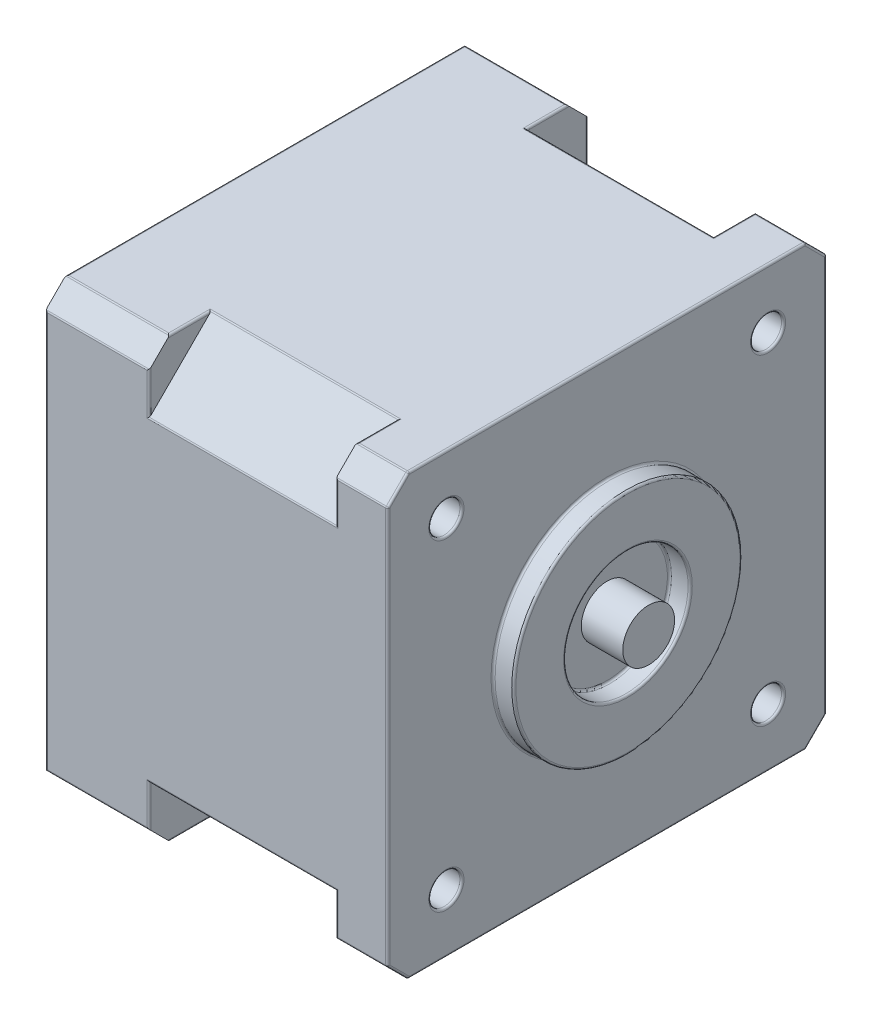
from build123d import *

# Parameters (mm, degrees)
BOSS_EXTRUDE1_DEPTH            = 5
BOSS_EXTRUDE2_DEPTH            = 18
BOSS_EXTRUDE3_DEPTH            = 10
BOSS_EXTRUDE4_DEPTH            = 2
SKETCH5_R                      = 11
BOSS_EXTRUDE5_DEPTH            = 2
F_12_0_12_DIAMETER_HOLE1_D     = 12.000000009
F_12_0_12_DIAMETER_HOLE1_DEPTH = 2
SKETCH8_W                      = 0.75
SKETCH8_H                      = 8
SKETCH9_W                      = 0.75
SKETCH9_H                      = 8
SKETCH10_W                     = 0.75
SKETCH10_H                     = 8
SKETCH11_W                     = 0.75
SKETCH11_H                     = 8
SKETCH12_W                     = 0.75
SKETCH12_H                     = 8
SKETCH13_W                     = 26
SKETCH13_H                     = 2.5
F_3_0_3_DIAMETER_HOLE1_D       = 2.999999994
F_3_0_3_DIAMETER_HOLE1_DEPTH   = 4.5
FILLET1_R                      = 0.2
SKETCH16_R                     = 3.097425191
CUT_EXTRUDE1_DEPTH             = 22


with BuildPart() as part:
    # Sketch1 → Boss-Extrude1 (new body)
    with BuildSketch(Plane(origin=(16.5, 0, 0), x_dir=(0, 0, -1), z_dir=(1, 0, 0))):
        Polygon((-21.15, 19.15), (-21.15, -19.15), (-19.15, -21.15), (19.15, -21.15), (21.15, -19.15), (21.15, 19.15), (19.15, 21.15), (-19.15, 21.15), align=None)
    extrude(amount=-BOSS_EXTRUDE1_DEPTH)

    # Sketch2 → Boss-Extrude2 (add)
    with BuildSketch(Plane.ZY.offset(-11.5)):
        Polygon((-15.15, 21.15), (15.15, 21.15), (21.15, 15.15), (21.15, -15.15), (15.15, -21.15), (-15.15, -21.15), (-21.15, -15.15), (-21.15, 15.15), align=None)
    extrude(amount=BOSS_EXTRUDE2_DEPTH)

    # Sketch3 → Boss-Extrude3 (add)
    with BuildSketch(Plane.ZY.offset(6.5)):
        Polygon((-19.15, -21.15), (-21.15, -19.15), (-21.15, 19.15), (-19.15, 21.15), (19.15, 21.15), (21.15, 19.15), (21.15, -19.15), (19.15, -21.15), align=None)
    extrude(amount=BOSS_EXTRUDE3_DEPTH)

    # Sketch4 → Boss-Extrude4 (add)
    with BuildSketch(Plane.XZ.offset(21.15)):
        with BuildLine():
            Line((-9.5, -5), (-14.5, -5))
            Line((-14.5, -5), (-14.5, 5))
            Line((-14.5, 5), (-9.5, 5))
            ThreePointArc((-9.5, 5), (-4.5, 0), (-9.5, -5))
        make_face()
    extrude(amount=BOSS_EXTRUDE4_DEPTH)

    # Sketch5 → Boss-Extrude5 (add)
    with BuildSketch(Plane(origin=(16.5, 0, 0), x_dir=(0, 0, -1), z_dir=(1, 0, 0))):
        Circle(SKETCH5_R)
    extrude(amount=BOSS_EXTRUDE5_DEPTH)

    # Ø12.0 (12) Diameter Hole1
    with Locations(Plane(origin=(18.5, 0, 0), x_dir=(0, 0, -1), z_dir=(1, 0, 0))):
        with Locations((0, 0)):
            Hole(F_12_0_12_DIAMETER_HOLE1_D / 2, depth=F_12_0_12_DIAMETER_HOLE1_DEPTH)

    # Sketch8 → Revolve1 (revolve)
    with BuildSketch(Plane.XY.offset(-4), mode=Mode.PRIVATE) as revolve1_sk:
        with Locations((-9.125, -27.15)):
            Rectangle(SKETCH8_W, SKETCH8_H)
    revolve(revolve1_sk.sketch.rotate(Axis((-9.5, -23.15, -4), (0, -1, 0)), 270), axis=Axis((-9.5, -23.15, -4), (0, -1, 0)))

    # Sketch9 → Revolve2 (revolve)
    with BuildSketch(Plane.XY.offset(-2), mode=Mode.PRIVATE) as revolve2_sk:
        with Locations((-9.125, -27.15)):
            Rectangle(SKETCH9_W, SKETCH9_H)
    revolve(revolve2_sk.sketch.rotate(Axis((-9.5, -23.15, -2), (0, -1, 0)), 270), axis=Axis((-9.5, -23.15, -2), (0, -1, 0)))

    # Sketch10 → Revolve3 (revolve)
    with BuildSketch(Plane.XY.offset(4), mode=Mode.PRIVATE) as revolve3_sk:
        with Locations((-9.125, -27.15)):
            Rectangle(SKETCH10_W, SKETCH10_H)
    revolve(revolve3_sk.sketch.rotate(Axis((-9.5, -23.15, 4), (0, -1, 0)), 270), axis=Axis((-9.5, -23.15, 4), (0, -1, 0)))

    # Sketch11 → Revolve4 (revolve)
    with BuildSketch(Plane.XY.offset(2), mode=Mode.PRIVATE) as revolve4_sk:
        with Locations((-9.125, -27.15)):
            Rectangle(SKETCH11_W, SKETCH11_H)
    revolve(revolve4_sk.sketch.rotate(Axis((-9.5, -23.15, 2), (0, -1, 0)), 270), axis=Axis((-9.5, -23.15, 2), (0, -1, 0)))

    # Sketch12 → Revolve5 (revolve)
    with BuildSketch(Plane.XY, mode=Mode.PRIVATE) as revolve5_sk:
        with Locations((-9.125, -27.15)):
            Rectangle(SKETCH12_W, SKETCH12_H)
    revolve(revolve5_sk.sketch.rotate(Axis((-9.5, -23.15, 0), (0, -1, 0)), 270), axis=Axis((-9.5, -23.15, 0), (0, -1, 0)))

    # Sketch13 → Revolve6 (revolve)
    with BuildSketch(Plane.XY, mode=Mode.PRIVATE) as revolve6_sk:
        with Locations((29.5, 1.25)):
            Rectangle(SKETCH13_W, SKETCH13_H)
    revolve(revolve6_sk.sketch.rotate(Axis((16.5, 0, 0), (1, 0, 0)), 270), axis=Axis((16.5, 0, 0), (1, 0, 0)))

    # Ø3.0 (3) Diameter Hole1
    with Locations(Plane(origin=(16.5, 0, 0), x_dir=(0, 0, -1), z_dir=(1, 0, 0))):
        with Locations((-15.5, 15.5), (15.5, -15.5), (15.5, 15.5), (-15.5, -15.5)):
            Hole(F_3_0_3_DIAMETER_HOLE1_D / 2, depth=F_3_0_3_DIAMETER_HOLE1_DEPTH)

    # Fillet1
    fillet1_edges = [part.edges().sort_by_distance(p)[0] for p in [
        (-16.5, 21.15, 0),
        (-11.5, 21.15, -19.15),
        (-11.5, 21.15, 19.15),
        (-6.5, 21.15, -17.15),
        (-11.5, 19.15, -21.15),
        (-16.5, 0, -21.15),
        (-16.5, 0, 21.15),
        (-6.5, 21.15, 17.15),
        (-11.5, 19.15, 21.15),
        (2.5, 21.15, -15.15),
        (-6.5, 17.15, -21.15),
        (-11.5, -19.15, -21.15),
        (-11.5, -19.15, 21.15),
        (2.5, 21.15, 15.15),
        (-6.5, 17.15, 21.15),
        (11.5, 21.15, -17.15),
        (2.5, 15.15, -21.15),
        (-6.5, -17.15, -21.15),
        (-6.5, -17.15, 21.15),
        (11.5, 21.15, 17.15),
        (2.5, 15.15, 21.15),
        (14, 21.15, -19.15),
        (11.5, 17.15, -21.15),
        (2.5, -15.15, -21.15),
        (2.5, -15.15, 21.15),
        (14, 21.15, 19.15),
        (16.5, 21.15, 0),
        (11.5, 17.15, 21.15),
        (2.5, -21.15, -15.15),
        (16.5, 20.15, -20.15),
        (14, 19.15, -21.15),
        (11.5, -17.15, -21.15),
        (11.5, -17.15, 21.15),
        (16.5, 20.15, 20.15),
        (14, 19.15, 21.15),
        (11.5, -21.15, -17.15),
        (16.5, 0, -21.15),
        (14, -19.15, -21.15),
        (14, -19.15, 21.15),
        (16.5, 0, 21.15),
        (14, -21.15, -19.15),
        (16.5, -20.15, -20.15),
        (16.5, -20.15, 20.15),
        (16.5, -21.15, 0),
        (14, -21.15, 19.15),
        (11.5, -21.15, 17.15),
        (2.5, -21.15, 15.15),
        (-6.5, -21.15, 17.15),
        (-11.5, -21.15, 19.15),
        (-16.5, -21.15, 0),
        (-11.5, -21.15, -19.15),
        (16.5, 0, -6.000000005),
        (18.5, 0, -6.000000005),
        (18.5, 0, 11),
        (-9.5, -31.15, 0.75),
        (-9.5, -31.15, 2.75),
        (-9.5, -31.15, 4.75),
        (-9.5, -31.15, -1.25),
        (-9.5, -31.15, -3.25),
        (16.5, 0, 11),
        (16.5, 15.5, 14.000000003),
        (16.5, -15.5, -16.999999997),
        (16.5, 15.5, -16.999999997),
        (16.5, -15.5, 14.000000003),
        (42.5, 0, 2.5),
        (-14.5, -23.15, 0),
        (-12, -23.15, 5),
        (-12, -23.15, -5),
        (-4.5, -23.15, 0),
    ]]
    fillet(fillet1_edges, radius=FILLET1_R)

    # Sketch16 → Cut-Extrude1 (cut)
    with BuildSketch(Plane(origin=(42.5, 0, 0), x_dir=(0, 0, -1), z_dir=(1, 0, 0))):
        Circle(SKETCH16_R)
    extrude(amount=-CUT_EXTRUDE1_DEPTH, mode=Mode.SUBTRACT)


solid = part.part
